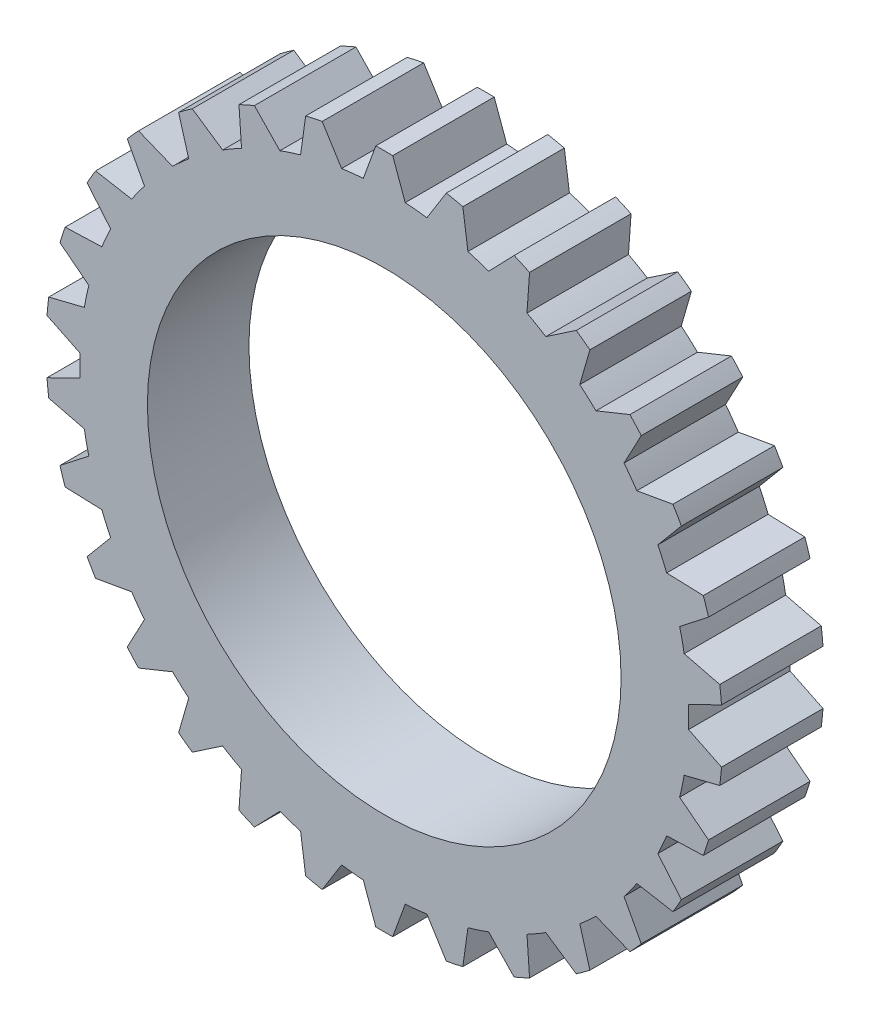
SolidWorks part; units mm, degrees
ref_plane "Front Plane" through (0, 0, 0) normal (0, 0, 1) x (1, 0, 0)
ref_plane "Top Plane" through (0, 0, 0) normal (0, 1, 0) x (1, 0, 0)
ref_plane "Right Plane" through (0, 0, 0) normal (1, 0, 0) x (0, 0, -1)
sketch "Sketch1" plane through (0, 0, 0) normal (0, 0, 1) x (1, 0, 0)
  line L0 (0, 0) -> (0, 100) construction
  line L1 (-2.5, 99.9687) -> (-6.2, 89.7862)
  line L2 (2.5, 99.9687) -> (6.2, 89.7862)
  line L3 (18.3393, 98.304) -> (12.6031, 89.1132)
  line L4 (23.23, 97.2644) -> (24.7321, 86.5351)
  line L5 (38.3771, 92.3428) -> (30.8554, 84.5455)
  line L6 (42.9448, 90.3092) -> (42.1833, 79.502)
  line L7 (56.7376, 82.3459) -> (47.7591, 76.2828)
  line L8 (60.7827, 79.407) -> (57.7909, 68.9943)
  line L9 (72.6184, 68.75) -> (62.5755, 64.6862)
  line L10 (75.9641, 65.0343) -> (70.8728, 55.4712)
  line L11 (85.3255, 52.1494) -> (74.6571, 50.2625)
  line L12 (87.8255, 47.8193) -> (80.8571, 39.5237)
  line L13 (94.3034, 33.2697) -> (83.4758, 33.642)
  line L14 (95.8485, 28.5144) -> (87.3076, 21.8489)
  line L15 (99.1598, 12.9359) -> (88.6463, 15.5512)
  line L16 (99.6824, 7.9633) -> (89.9424, 3.2192)
  line L17 (99.6824, -7.9633) -> (89.9424, -3.2192)
  line L18 (99.1598, -12.9359) -> (88.6463, -15.5512)
  line L19 (95.8485, -28.5144) -> (87.3076, -21.8489)
  line L20 (94.3034, -33.2697) -> (83.4758, -33.642)
  line L21 (87.8255, -47.8193) -> (80.8571, -39.5237)
  line L22 (85.3255, -52.1494) -> (74.6571, -50.2625)
  line L23 (75.9641, -65.0343) -> (70.8728, -55.4712)
  line L24 (72.6184, -68.75) -> (62.5755, -64.6862)
  line L25 (60.7827, -79.407) -> (57.7909, -68.9943)
  line L26 (56.7376, -82.3459) -> (47.7591, -76.2828)
  line L27 (42.9448, -90.3092) -> (42.1833, -79.502)
  line L28 (38.3771, -92.3428) -> (30.8554, -84.5455)
  line L29 (23.23, -97.2644) -> (24.7321, -86.5351)
  line L30 (18.3393, -98.304) -> (12.6031, -89.1132)
  line L31 (2.5, -99.9687) -> (6.2, -89.7862)
  line L32 (-2.5, -99.9687) -> (-6.2, -89.7862)
  line L33 (-18.3393, -98.304) -> (-12.6031, -89.1132)
  line L34 (-23.23, -97.2644) -> (-24.7321, -86.5351)
  line L35 (-38.3771, -92.3428) -> (-30.8554, -84.5455)
  line L36 (-42.9448, -90.3092) -> (-42.1833, -79.502)
  line L37 (-56.7376, -82.3459) -> (-47.7591, -76.2828)
  line L38 (-60.7827, -79.407) -> (-57.7909, -68.9943)
  line L39 (-72.6184, -68.75) -> (-62.5755, -64.6862)
  line L40 (-75.9641, -65.0343) -> (-70.8728, -55.4712)
  line L41 (-85.3255, -52.1494) -> (-74.6571, -50.2625)
  line L42 (-87.8255, -47.8193) -> (-80.8571, -39.5237)
  line L43 (-94.3034, -33.2697) -> (-83.4758, -33.642)
  line L44 (-95.8485, -28.5144) -> (-87.3076, -21.8489)
  line L45 (-99.1598, -12.9359) -> (-88.6463, -15.5512)
  line L46 (-99.6824, -7.9633) -> (-89.9424, -3.2192)
  line L47 (-99.6824, 7.9633) -> (-89.9424, 3.2192)
  line L48 (-99.1598, 12.9359) -> (-88.6463, 15.5512)
  line L49 (-95.8485, 28.5144) -> (-87.3076, 21.8489)
  line L50 (-94.3034, 33.2697) -> (-83.4758, 33.642)
  line L51 (-87.8255, 47.8193) -> (-80.8571, 39.5237)
  line L52 (-85.3255, 52.1494) -> (-74.6571, 50.2625)
  line L53 (-75.9641, 65.0343) -> (-70.8728, 55.4712)
  line L54 (-72.6184, 68.75) -> (-62.5755, 64.6862)
  line L55 (-60.7827, 79.407) -> (-57.7909, 68.9943)
  line L56 (-56.7376, 82.3459) -> (-47.7591, 76.2828)
  line L57 (-42.9448, 90.3092) -> (-42.1833, 79.502)
  line L58 (-38.3771, 92.3428) -> (-30.8554, 84.5455)
  line L59 (-23.23, 97.2644) -> (-24.7321, 86.5351)
  line L60 (-18.3393, 98.304) -> (-12.6031, 89.1132)
  line L65 (-21.9549, 97.5601) -> (-23.5973, 86.8514) [skipped]
  line L66 (-40.5661, 91.4024) -> (-40.0877, 80.579) [skipped]
  line L67 (-57.6183, 81.732) -> (-55.0376, 71.21) [skipped]
  line L68 (-72.4563, 68.9208) -> (-67.8725, 59.1044) [skipped]
  line L69 (-84.5099, 53.461) -> (-78.099, 44.7274) [skipped]
  line L70 (35.9467, 93.3158) -> (28.6316, 85.3243) [skipped]
  line L71 (53.461, 84.5099) -> (44.7274, 78.099) [skipped]
  line L72 (68.9208, 72.4563) -> (59.1044, 67.8725) [skipped]
  line L73 (81.732, 57.6183) -> (71.21, 55.0376) [skipped]
  line L74 (91.4024, 40.5661) -> (80.579, 40.0877) [skipped]
  line L75 (97.5601, 21.9549) -> (86.8514, 23.5973) [skipped]
  line L76 (99.9687, 2.5) -> (89.7862, 6.2) [skipped]
  line L77 (98.5356, -17.051) -> (89.2705, -11.4355) [skipped]
  line L78 (93.3158, -35.9467) -> (85.3243, -28.6316) [skipped]
  line L79 (84.5099, -53.461) -> (78.099, -44.7274) [skipped]
  line L80 (40.5661, -91.4024) -> (40.0877, -80.579) [skipped]
  line L81 (21.9549, -97.5601) -> (23.5973, -86.8514) [skipped]
  line L82 (2.5, -99.9687) -> (6.2, -89.7862) [skipped]
  line L83 (-17.051, -98.5356) -> (-11.4355, -89.2705) [skipped]
  line L84 (72.4563, -68.9208) -> (67.8725, -59.1044) [skipped]
  line L85 (57.6183, -81.732) -> (55.0376, -71.21) [skipped]
  line L86 (-81.732, -57.6183) -> (-71.21, -55.0376) [skipped]
  line L87 (-91.4024, -40.5661) -> (-80.579, -40.0877) [skipped]
  line L88 (-97.5601, -21.9549) -> (-86.8514, -23.5973) [skipped]
  line L89 (-99.9687, -2.5) -> (-89.7862, -6.2) [skipped]
  line L90 (-35.9467, -93.3158) -> (-28.6316, -85.3243) [skipped]
  line L91 (-53.461, -84.5099) -> (-44.7274, -78.099) [skipped]
  line L92 (-68.9208, -72.4563) -> (-59.1044, -67.8725) [skipped]
  line L93 (-98.5356, 17.051) -> (-89.2705, 11.4355) [skipped]
  line L94 (-93.3158, 35.9467) -> (-85.3243, 28.6316) [skipped]
  line L95 (17.051, 98.5356) -> (11.4355, 89.2705) [skipped]
  arc A1 (-2.5, 99.9687) -> (2.5, 99.9687) centre (0, 0) cw
  arc A2 (-42.1833, 79.502) -> (-47.7591, 76.2828) centre (0, 0) ccw construction
  arc A3 (18.3393, 98.304) -> (23.23, 97.2644) centre (0, 0) cw
  arc A4 (38.3771, 92.3428) -> (42.9448, 90.3092) centre (0, 0) cw
  arc A5 (56.7376, 82.3459) -> (60.7827, 79.407) centre (0, 0) cw
  arc A6 (72.6184, 68.75) -> (75.9641, 65.0343) centre (0, 0) cw
  arc A7 (85.3255, 52.1494) -> (87.8255, 47.8193) centre (0, 0) cw
  arc A8 (94.3034, 33.2697) -> (95.8485, 28.5144) centre (0, 0) cw
  arc A9 (99.1598, 12.9359) -> (99.6824, 7.9633) centre (0, 0) cw
  arc A10 (99.6824, -7.9633) -> (99.1598, -12.9359) centre (0, 0) cw
  arc A11 (95.8485, -28.5144) -> (94.3034, -33.2697) centre (0, 0) cw
  arc A12 (87.8255, -47.8193) -> (85.3255, -52.1494) centre (0, 0) cw
  arc A13 (75.9641, -65.0343) -> (72.6184, -68.75) centre (0, 0) cw
  arc A14 (60.7827, -79.407) -> (56.7376, -82.3459) centre (0, 0) cw
  arc A15 (42.9448, -90.3092) -> (38.3771, -92.3428) centre (0, 0) cw
  arc A16 (23.23, -97.2644) -> (18.3393, -98.304) centre (0, 0) cw
  arc A17 (2.5, -99.9687) -> (-2.5, -99.9687) centre (0, 0) cw
  arc A18 (-18.3393, -98.304) -> (-23.23, -97.2644) centre (0, 0) cw
  arc A19 (-38.3771, -92.3428) -> (-42.9448, -90.3092) centre (0, 0) cw
  arc A20 (-56.7376, -82.3459) -> (-60.7827, -79.407) centre (0, 0) cw
  arc A21 (-72.6184, -68.75) -> (-75.9641, -65.0343) centre (0, 0) cw
  arc A22 (-85.3255, -52.1494) -> (-87.8255, -47.8193) centre (0, 0) cw
  arc A23 (-94.3034, -33.2697) -> (-95.8485, -28.5144) centre (0, 0) cw
  arc A24 (-99.1598, -12.9359) -> (-99.6824, -7.9633) centre (0, 0) cw
  arc A25 (-99.6824, 7.9633) -> (-99.1598, 12.9359) centre (0, 0) cw
  arc A26 (-95.8485, 28.5144) -> (-94.3034, 33.2697) centre (0, 0) cw
  arc A27 (-87.8255, 47.8193) -> (-85.3255, 52.1494) centre (0, 0) cw
  arc A28 (-75.9641, 65.0343) -> (-72.6184, 68.75) centre (0, 0) cw
  arc A29 (-60.7827, 79.407) -> (-56.7376, 82.3459) centre (0, 0) cw
  arc A30 (-42.9448, 90.3092) -> (-38.3771, 92.3428) centre (0, 0) cw
  arc A31 (-23.23, 97.2644) -> (-18.3393, 98.304) centre (0, 0) cw
  arc A32 (-42.1833, 79.502) -> (-47.7591, 76.2828) centre (0, 0) ccw
  arc A33 (-57.7909, 68.9943) -> (-62.5755, 64.6862) centre (0, 0) ccw construction
  arc A34 (-57.7909, 68.9943) -> (-62.5755, 64.6862) centre (0, 0) ccw
  arc A35 (-70.8728, 55.4712) -> (-74.6571, 50.2625) centre (0, 0) ccw construction
  arc A36 (-70.8728, 55.4712) -> (-74.6571, 50.2625) centre (0, 0) ccw
  arc A37 (-80.8571, 39.5237) -> (-83.4758, 33.642) centre (0, 0) ccw construction
  arc A38 (-80.8571, 39.5237) -> (-83.4758, 33.642) centre (0, 0) ccw
  arc A39 (-87.3076, 21.8489) -> (-88.6463, 15.5512) centre (0, 0) ccw construction
  arc A40 (-87.3076, 21.8489) -> (-88.6463, 15.5512) centre (0, 0) ccw
  arc A41 (-89.9424, 3.2192) -> (-89.9424, -3.2192) centre (0, 0) ccw construction
  arc A42 (-89.9424, 3.2192) -> (-89.9424, -3.2192) centre (0, 0) ccw
  arc A43 (-88.6463, -15.5512) -> (-87.3076, -21.8489) centre (0, 0) ccw construction
  arc A44 (-88.6463, -15.5512) -> (-87.3076, -21.8489) centre (0, 0) ccw
  arc A45 (-83.4758, -33.642) -> (-80.8571, -39.5237) centre (0, 0) ccw construction
  arc A46 (-83.4758, -33.642) -> (-80.8571, -39.5237) centre (0, 0) ccw
  arc A47 (-74.6571, -50.2625) -> (-70.8728, -55.4712) centre (0, 0) ccw construction
  arc A48 (-74.6571, -50.2625) -> (-70.8728, -55.4712) centre (0, 0) ccw
  arc A49 (-62.5755, -64.6862) -> (-57.7909, -68.9943) centre (0, 0) ccw construction
  arc A50 (-62.5755, -64.6862) -> (-57.7909, -68.9943) centre (0, 0) ccw
  arc A51 (-47.7591, -76.2828) -> (-42.1833, -79.502) centre (0, 0) ccw construction
  arc A52 (-47.7591, -76.2828) -> (-42.1833, -79.502) centre (0, 0) ccw
  arc A53 (-30.8554, -84.5455) -> (-24.7321, -86.5351) centre (0, 0) ccw construction
  arc A54 (-12.6031, -89.1132) -> (-6.2, -89.7862) centre (0, 0) ccw
  arc A55 (-12.6031, -89.1132) -> (-6.2, -89.7862) centre (0, 0) ccw construction
  arc A56 (-30.8554, -84.5455) -> (-24.7321, -86.5351) centre (0, 0) ccw
  arc A57 (6.2, -89.7862) -> (12.6031, -89.1132) centre (0, 0) ccw
  arc A58 (6.2, -89.7862) -> (12.6031, -89.1132) centre (0, 0) ccw construction
  arc A59 (24.7321, -86.5351) -> (30.8554, -84.5455) centre (0, 0) ccw
  arc A60 (24.7321, -86.5351) -> (30.8554, -84.5455) centre (0, 0) ccw construction
  arc A61 (42.1833, -79.502) -> (47.7591, -76.2828) centre (0, 0) ccw
  arc A62 (42.1833, -79.502) -> (47.7591, -76.2828) centre (0, 0) ccw construction
  arc A63 (57.7909, -68.9943) -> (62.5755, -64.6862) centre (0, 0) ccw
  circle A64 centre (0, 0) radius 70
  arc A65 (35.9467, 93.3158) -> (40.5661, 91.4024) centre (0, 0) cw [skipped]
  arc A66 (53.461, 84.5099) -> (57.6183, 81.732) centre (0, 0) cw [skipped]
  arc A67 (68.9208, 72.4563) -> (72.4563, 68.9208) centre (0, 0) cw [skipped]
  arc A68 (81.732, 57.6183) -> (84.5099, 53.461) centre (0, 0) cw [skipped]
  arc A69 (91.4024, 40.5661) -> (93.3158, 35.9467) centre (0, 0) cw [skipped]
  arc A70 (97.5601, 21.9549) -> (98.5356, 17.051) centre (0, 0) cw [skipped]
  arc A71 (99.9687, 2.5) -> (99.9687, -2.5) centre (0, 0) cw [skipped]
  arc A72 (98.5356, -17.051) -> (97.5601, -21.9549) centre (0, 0) cw [skipped]
  arc A73 (93.3158, -35.9467) -> (91.4024, -40.5661) centre (0, 0) cw [skipped]
  arc A74 (84.5099, -53.461) -> (81.732, -57.6183) centre (0, 0) cw [skipped]
  arc A75 (57.6183, -81.732) -> (53.461, -84.5099) centre (0, 0) cw [skipped]
  arc A76 (40.5661, -91.4024) -> (35.9467, -93.3158) centre (0, 0) cw [skipped]
  arc A77 (21.9549, -97.5601) -> (17.051, -98.5356) centre (0, 0) cw [skipped]
  arc A78 (2.5, -99.9687) -> (-2.5, -99.9687) centre (0, 0) cw [skipped]
  arc A79 (-17.051, -98.5356) -> (-21.9549, -97.5601) centre (0, 0) cw [skipped]
  arc A80 (72.4563, -68.9208) -> (68.9208, -72.4563) centre (0, 0) cw [skipped]
  arc A81 (-81.732, -57.6183) -> (-84.5099, -53.461) centre (0, 0) cw [skipped]
  arc A82 (-91.4024, -40.5661) -> (-93.3158, -35.9467) centre (0, 0) cw [skipped]
  arc A83 (-97.5601, -21.9549) -> (-98.5356, -17.051) centre (0, 0) cw [skipped]
  arc A84 (-99.9687, -2.5) -> (-99.9687, 2.5) centre (0, 0) cw [skipped]
  arc A85 (-35.9467, -93.3158) -> (-40.5661, -91.4024) centre (0, 0) cw [skipped]
  arc A86 (-53.461, -84.5099) -> (-57.6183, -81.732) centre (0, 0) cw [skipped]
  arc A87 (-68.9208, -72.4563) -> (-72.4563, -68.9208) centre (0, 0) cw [skipped]
  arc A88 (-98.5356, 17.051) -> (-97.5601, 21.9549) centre (0, 0) cw [skipped]
  arc A89 (-93.3158, 35.9467) -> (-91.4024, 40.5661) centre (0, 0) cw [skipped]
  arc A90 (-84.5099, 53.461) -> (-81.732, 57.6183) centre (0, 0) cw [skipped]
  arc A91 (-72.4563, 68.9208) -> (-68.9208, 72.4563) centre (0, 0) cw [skipped]
  arc A92 (-57.6183, 81.732) -> (-53.461, 84.5099) centre (0, 0) cw [skipped]
  arc A93 (-40.5661, 91.4024) -> (-35.9467, 93.3158) centre (0, 0) cw [skipped]
  arc A94 (-21.9549, 97.5601) -> (-17.051, 98.5356) centre (0, 0) cw [skipped]
  arc A95 (17.051, 98.5356) -> (21.9549, 97.5601) centre (0, 0) cw [skipped]
  arc A96 (57.7909, -68.9943) -> (62.5755, -64.6862) centre (0, 0) ccw construction
  arc A97 (80.8571, -39.5237) -> (83.4758, -33.642) centre (0, 0) ccw
  arc A98 (80.8571, -39.5237) -> (83.4758, -33.642) centre (0, 0) ccw construction
  arc A99 (87.3076, -21.8489) -> (88.6463, -15.5512) centre (0, 0) ccw
  arc A100 (87.3076, -21.8489) -> (88.6463, -15.5512) centre (0, 0) ccw construction
  arc A101 (70.8728, -55.4712) -> (74.6571, -50.2625) centre (0, 0) ccw
  arc A102 (70.8728, -55.4712) -> (74.6571, -50.2625) centre (0, 0) ccw construction
  arc A103 (89.9424, -3.2192) -> (89.9424, 3.2192) centre (0, 0) ccw
  arc A104 (89.9424, -3.2192) -> (89.9424, 3.2192) centre (0, 0) ccw construction
  arc A105 (88.6463, 15.5512) -> (87.3076, 21.8489) centre (0, 0) ccw
  arc A106 (88.6463, 15.5512) -> (87.3076, 21.8489) centre (0, 0) ccw construction
  arc A107 (83.4758, 33.642) -> (80.8571, 39.5237) centre (0, 0) ccw
  arc A108 (83.4758, 33.642) -> (80.8571, 39.5237) centre (0, 0) ccw construction
  arc A109 (74.6571, 50.2625) -> (70.8728, 55.4712) centre (0, 0) ccw
  arc A110 (74.6571, 50.2625) -> (70.8728, 55.4712) centre (0, 0) ccw construction
  arc A111 (62.5755, 64.6862) -> (57.7909, 68.9943) centre (0, 0) ccw
  arc A112 (62.5755, 64.6862) -> (57.7909, 68.9943) centre (0, 0) ccw construction
  arc A113 (47.7591, 76.2828) -> (42.1833, 79.502) centre (0, 0) ccw
  arc A114 (47.7591, 76.2828) -> (42.1833, 79.502) centre (0, 0) ccw construction
  arc A115 (30.8554, 84.5455) -> (24.7321, 86.5351) centre (0, 0) ccw
  arc A116 (30.8554, 84.5455) -> (24.7321, 86.5351) centre (0, 0) ccw construction
  arc A117 (12.6031, 89.1132) -> (6.2, 89.7862) centre (0, 0) ccw
  arc A118 (12.6031, 89.1132) -> (6.2, 89.7862) centre (0, 0) ccw construction
  arc A119 (-6.2, 89.7862) -> (-12.6031, 89.1132) centre (0, 0) ccw
  arc A120 (-6.2, 89.7862) -> (-12.6031, 89.1132) centre (0, 0) ccw construction
  arc A121 (-24.7321, 86.5351) -> (-30.8554, 84.5455) centre (0, 0) ccw
  arc A122 (-24.7321, 86.5351) -> (-30.8554, 84.5455) centre (0, 0) ccw construction
  point P4 (0, 100)
  point P8 (0, 0)
  point P130 (0, 0)
  point P169 (0, 0)
  dimension "D1" = 180
  dimension "D2" = 100
  dimension "D8" = 140
  dimension "D3" = 2.5
  dimension "D4" = 30
  dimension "D5" = 6.2
  dimension "D6" = 6.2
  dimension "D7" = 32
extrude "Boss-Extrude1" add sketch "Sketch1" along normal blind 30
sketch "Sketch2" plane through (0, 0, 30) normal (0, 0, 1) x (1, 0, 0)
  line L2 (-42.9448, 90.3092) -> (-42.1833, 79.502) construction
  circle A0 centre (0, 0) radius 94.9771
  point P8 (-42.5641, 84.9056)
